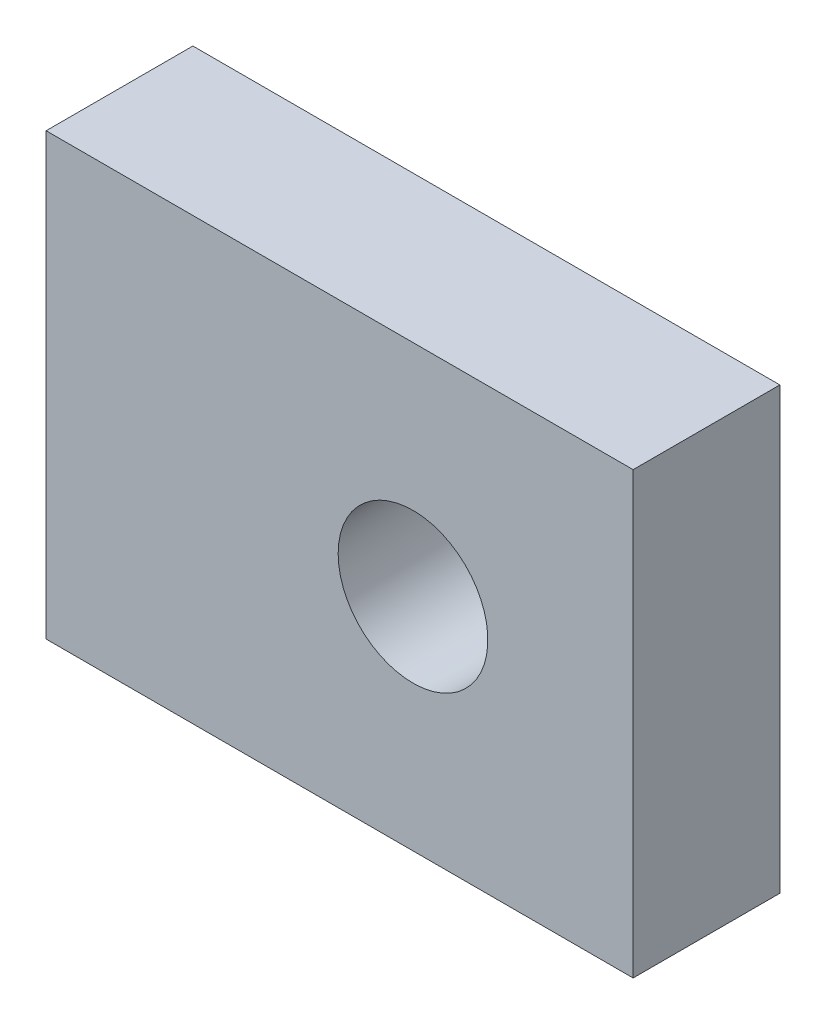
SolidWorks part; units mm, degrees
material "Q235B"
ref_plane "Front Plane" through (0, 0, 0) normal (0, 0, 1) x (1, 0, 0)
ref_plane "Top Plane" through (0, 0, 0) normal (0, 1, 0) x (1, 0, 0)
ref_plane "Right Plane" through (0, 0, 0) normal (1, 0, 0) x (0, 0, -1)
other "Configuration Table"
sketch "Sketch1" plane through (0, 0, 0) normal (0, 0, 1) x (1, 0, 0)
  line L1 (-20, -15) -> (20, -15)
  line L2 (-20, -15) -> (-20, 15)
  line L3 (-20, 15) -> (20, 15)
  line L4 (20, -15) -> (20, 15)
  line L5 (-20, -15) -> (20, 15) construction
  line L6 (-20, 15) -> (20, -15) construction
  circle A0 centre (5, 0) radius 5
  point P0 (0, 0)
  dimension "D4" = 10
  dimension "D1" = 40
  dimension "D2" = 30
  dimension "D3" = 15
  dimension "D5" = 0
extrude "Boss-Extrude1" add sketch "Sketch1" along normal blind 10
hole_wizard "M12 Tapped Hole1" positions "3DSketch1" profile "Sketch3" tap size "M12" standard "GB" end condition through all
sketch3d "3DSketch1"
  line L0 (5, 0, 10) -> (5, 0, 0) construction
  point P0 (5, 0, 0)
sketch "Sketch3" plane through (5, 0, 0) normal (1, 0, 0) x (0, 1, 0)
  line L0 (0, 0) -> (0, 10)
  line L1 (0, 10) -> (5.1, 10)
  line L2 (5.1, 10) -> (5.1, 0)
  line L5 (5.1, 0) -> (0, 0)
  line L11 (0, -6.35) -> (0, 107.95) construction
  dimension "通孔螺纹孔钻头直径" = 10.2
  dimension "通孔螺纹孔钻头深度" = 10
cosmetic thread "Cosmetic thread1" parameters "D2"=12
